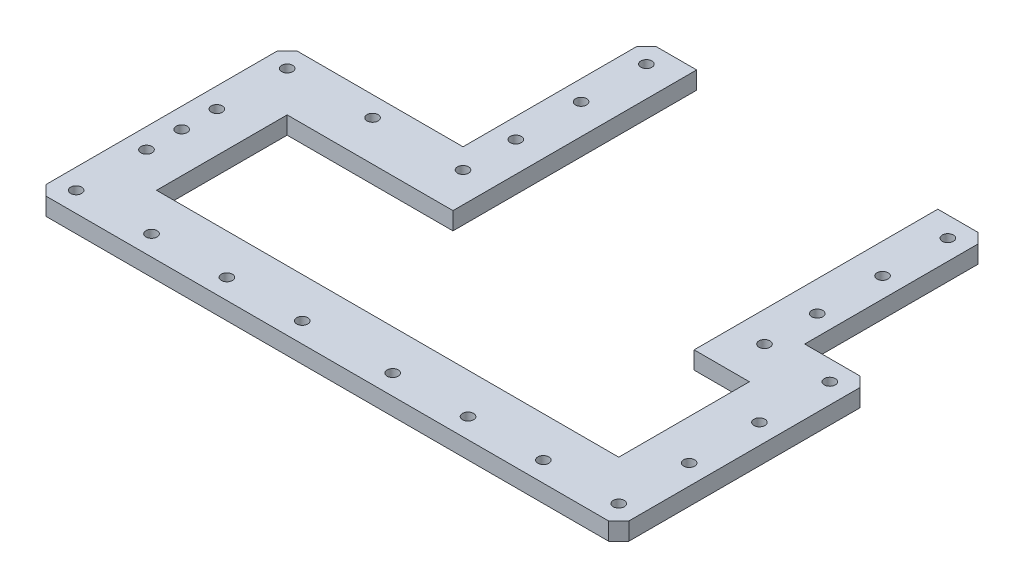
SolidWorks part; units mm, degrees
ref_plane "Front Plane" through (0, 0, 0) normal (0, 0, 1) x (1, 0, 0)
ref_plane "Top Plane" through (0, 0, 0) normal (0, 1, 0) x (1, 0, 0)
ref_plane "Right Plane" through (0, 0, 0) normal (1, 0, 0) x (0, 0, -1)
sketch "Sketch1" plane through (0, 0, 0) normal (0, 1, 0) x (1, 0, 0)
  line L0 (-1160, 500) -> (-810, 500)
  line L1 (0, 0) -> (-1160, 0)
  line L2 (0, 0) -> (0, 500)
  line L3 (-130, 865) -> (-230, 865)
  line L4 (-1160, 0) -> (-1160, 500)
  line L5 (-810, 500) -> (-810, 865)
  line L6 (-130, 865) -> (-130, 500)
  line L7 (-130, 500) -> (0, 500)
  line L8 (-710, 865) -> (-710, 745)
  line L9 (-470, 1014.2039) -> (-470, -321.2652) construction
  line L10 (-230, 865) -> (-230, 745)
  line L11 (-710, 745) -> (-230, 745)
  line L12 (-710, 865) -> (-810, 865)
  point P15 (-230, 805)
  dimension "D1" = 1160
  dimension "D2" = 500
  dimension "D3" = 365
  dimension "D4" = 100
  dimension "D5" = 100
  dimension "D6" = 450
  dimension "D7" = 230
  dimension "D8" = 120
extrude "Boss-Extrude1" add sketch "Sketch1" along normal blind 35
sketch "Sketch4" plane through (0, 35, 0) normal (0, 1, 0) x (1, 0, 0)
  line L18 (-1160, 500) -> (-1160, 0)
  line L19 (-1040, 120) -> (-120, 120)
  line L20 (-1160, 0) -> (0, 0)
  line L21 (-120, 120) -> (-120, 380)
  line L22 (0, 0) -> (0, 500)
  line L23 (-120, 380) -> (-250, 380)
  line L24 (0, 500) -> (-130, 500)
  line L25 (-130, 500) -> (-130, 865)
  line L27 (-130, 865) -> (-230, 865)
  line L28 (-230, 865) -> (-230, 745)
  line L29 (-230, 745) -> (-710, 745)
  line L30 (-710, 745) -> (-710, 865)
  line L31 (-710, 865) -> (-810, 865)
  line L33 (-810, 865) -> (-810, 500)
  line L34 (-810, 500) -> (-1160, 500)
  line L38 (-1160, 0) -> (0, 0)
  line L58 (-690, 380) -> (-1040, 380)
  line L59 (-1040, 380) -> (-1040, 120)
  line L60 (0, 0) -> (0, 500)
  line L61 (0, 500) -> (-130, 500)
  line L62 (-130, 500) -> (-130, 865)
  line L63 (-130, 865) -> (-230, 865)
  line L64 (-230, 865) -> (-230, 745)
  line L65 (-230, 745) -> (-710, 745)
  line L66 (-710, 745) -> (-710, 865)
  line L67 (-710, 865) -> (-810, 865)
  line L68 (-810, 865) -> (-810, 500)
  line L69 (-810, 500) -> (-1160, 500)
  line L70 (-1160, 500) -> (-1160, 0)
  line L71 (-1160, 0) -> (0, 0)
  line L72 (0, 0) -> (0, 500) construction
  line L73 (0, 500) -> (-130, 500) construction
  line L74 (-130, 500) -> (-130, 865) construction
  line L75 (-130, 865) -> (-230, 865) construction
  line L76 (-230, 865) -> (-230, 745) construction
  line L77 (-230, 745) -> (-710, 745) construction
  line L78 (-710, 745) -> (-710, 865) construction
  line L79 (-710, 865) -> (-810, 865) construction
  line L80 (-810, 865) -> (-810, 500) construction
  line L81 (-810, 500) -> (-1160, 500) construction
  line L82 (-1160, 500) -> (-1160, 0) construction
  line L83 (-1160, 0) -> (0, 0) construction
  line L84 (-1040, 120) -> (-120, 120)
  line L85 (-1160, 120) -> (0, 120) construction
  line L86 (-710, 380) -> (-710, 775)
  line L87 (-710, 775) -> (-230, 775)
  line L88 (-230, 775) -> (-230, 380)
  line L103 (-250, 625) -> (-690, 625) construction
  line L104 (-690, 625) -> (-690, 380) construction
  line L105 (-250, 380) -> (-250, 625) construction
  line L106 (-250, 625) -> (-250, 625) construction
  line L107 (-250, 625) -> (-250, 625) construction
  line L108 (-690, 625) -> (-690, 625) construction
  line L109 (-690, 625) -> (-690, 625) construction
  dimension "D3" = 120
  dimension "D4" = 100
  dimension "D5" = 100
  dimension "D6" = 90
  dimension "D1" = 0
  dimension "D2" = 0
extrude "Cut-Extrude1" cut sketch "Sketch4" against normal through all and the other way through all
sketch "Sketch5" plane through (0, 35, 0) normal (0, 1, 0) x (1, 0, 0)
  line L0 (-1160, 500) -> (-1160, 0) construction
  line L1 (-1160, 40) -> (0, 40) construction
  line L2 (0, 0) -> (0, 500) construction
  line L3 (-1160, 0) -> (0, 0) construction
  line L4 (-770, 1019.7156) -> (-770, -173.41) construction
  line L5 (-950, 997.2884) -> (-950, -278.8177) construction
  line L6 (-710, 865) -> (-230, 865) construction
  line L7 (-470, 1035.2394) -> (-470, -318.0992) construction
  line L8 (-710, 380) -> (-710, 865) construction
  line L9 (-1120, 997.2884) -> (-1120, -206.0693) construction
  line L10 (-1120, 460) -> (-710, 460) construction
  line L11 (-710, 380) -> (-710, 865) construction
  line L12 (-40, 460) -> (-40, 0) construction
  circle A0 centre (-1120, 40) radius 11
  circle A2 centre (-970, 40) radius 11
  circle A3 centre (-820, 40) radius 11
  circle A4 centre (-670, 40) radius 11
  circle A5 centre (-490, 40) radius 11
  circle A6 centre (-340, 40) radius 11
  circle A7 centre (-190, 40) radius 11
  circle A8 centre (-40, 40) radius 11
  circle A9 centre (-770, 825) radius 11
  circle A10 centre (-770, 695) radius 11
  circle A11 centre (-770, 565) radius 11
  circle A12 centre (-770, 460) radius 11
  circle A13 centre (-1120, 180) radius 11
  circle A14 centre (-1120, 250) radius 11
  circle A15 centre (-1120, 320) radius 11
  circle A16 centre (-1120, 460) radius 11
  circle A17 centre (-950, 460) radius 11
  circle A18 centre (-170, 460) radius 11
  circle A19 centre (-170, 565) radius 11
  circle A20 centre (-170, 695) radius 11
  circle A21 centre (-170, 825) radius 11
  circle A22 centre (-40, 460) radius 11
  circle A23 centre (-40, 320) radius 11
  circle A24 centre (-40, 180) radius 11
  dimension "D1" = 22
  dimension "D5" = 40
  dimension "D8" = 22
  dimension "D14" = 22
  dimension "D2" = 40
  dimension "D4" = 150
  dimension "D6" = 180
  dimension "D9" = 150
  dimension "D10" = 240
  dimension "D11" = 300
  dimension "D12" = 180
  dimension "D13" = 170
  dimension "D15" = 140
  dimension "D16" = 70
  dimension "D17" = 70
  dimension "D18" = 140
  dimension "D19" = 105
  dimension "D20" = 130
  dimension "D21" = 130
  dimension "D22" = 105
  dimension "D23" = 140
  dimension "D24" = 140
  dimension "D25" = 140
  dimension "D26" = 130
  dimension "D27" = 130
  dimension "D3" = 4
  dimension "D7" = 4
chamfer "Chamfer2" distance 20 angle 45 6 edges at (-1160, 17.5, 0) (0, 17.5, 0) (0, 17.5, -500) (-130, 17.5, -865) (-810, 17.5, -865) (-1160, 17.5, -500)
extrude "Cut-Extrude2" cut sketch "Sketch5" against normal through all both and the other way through all
